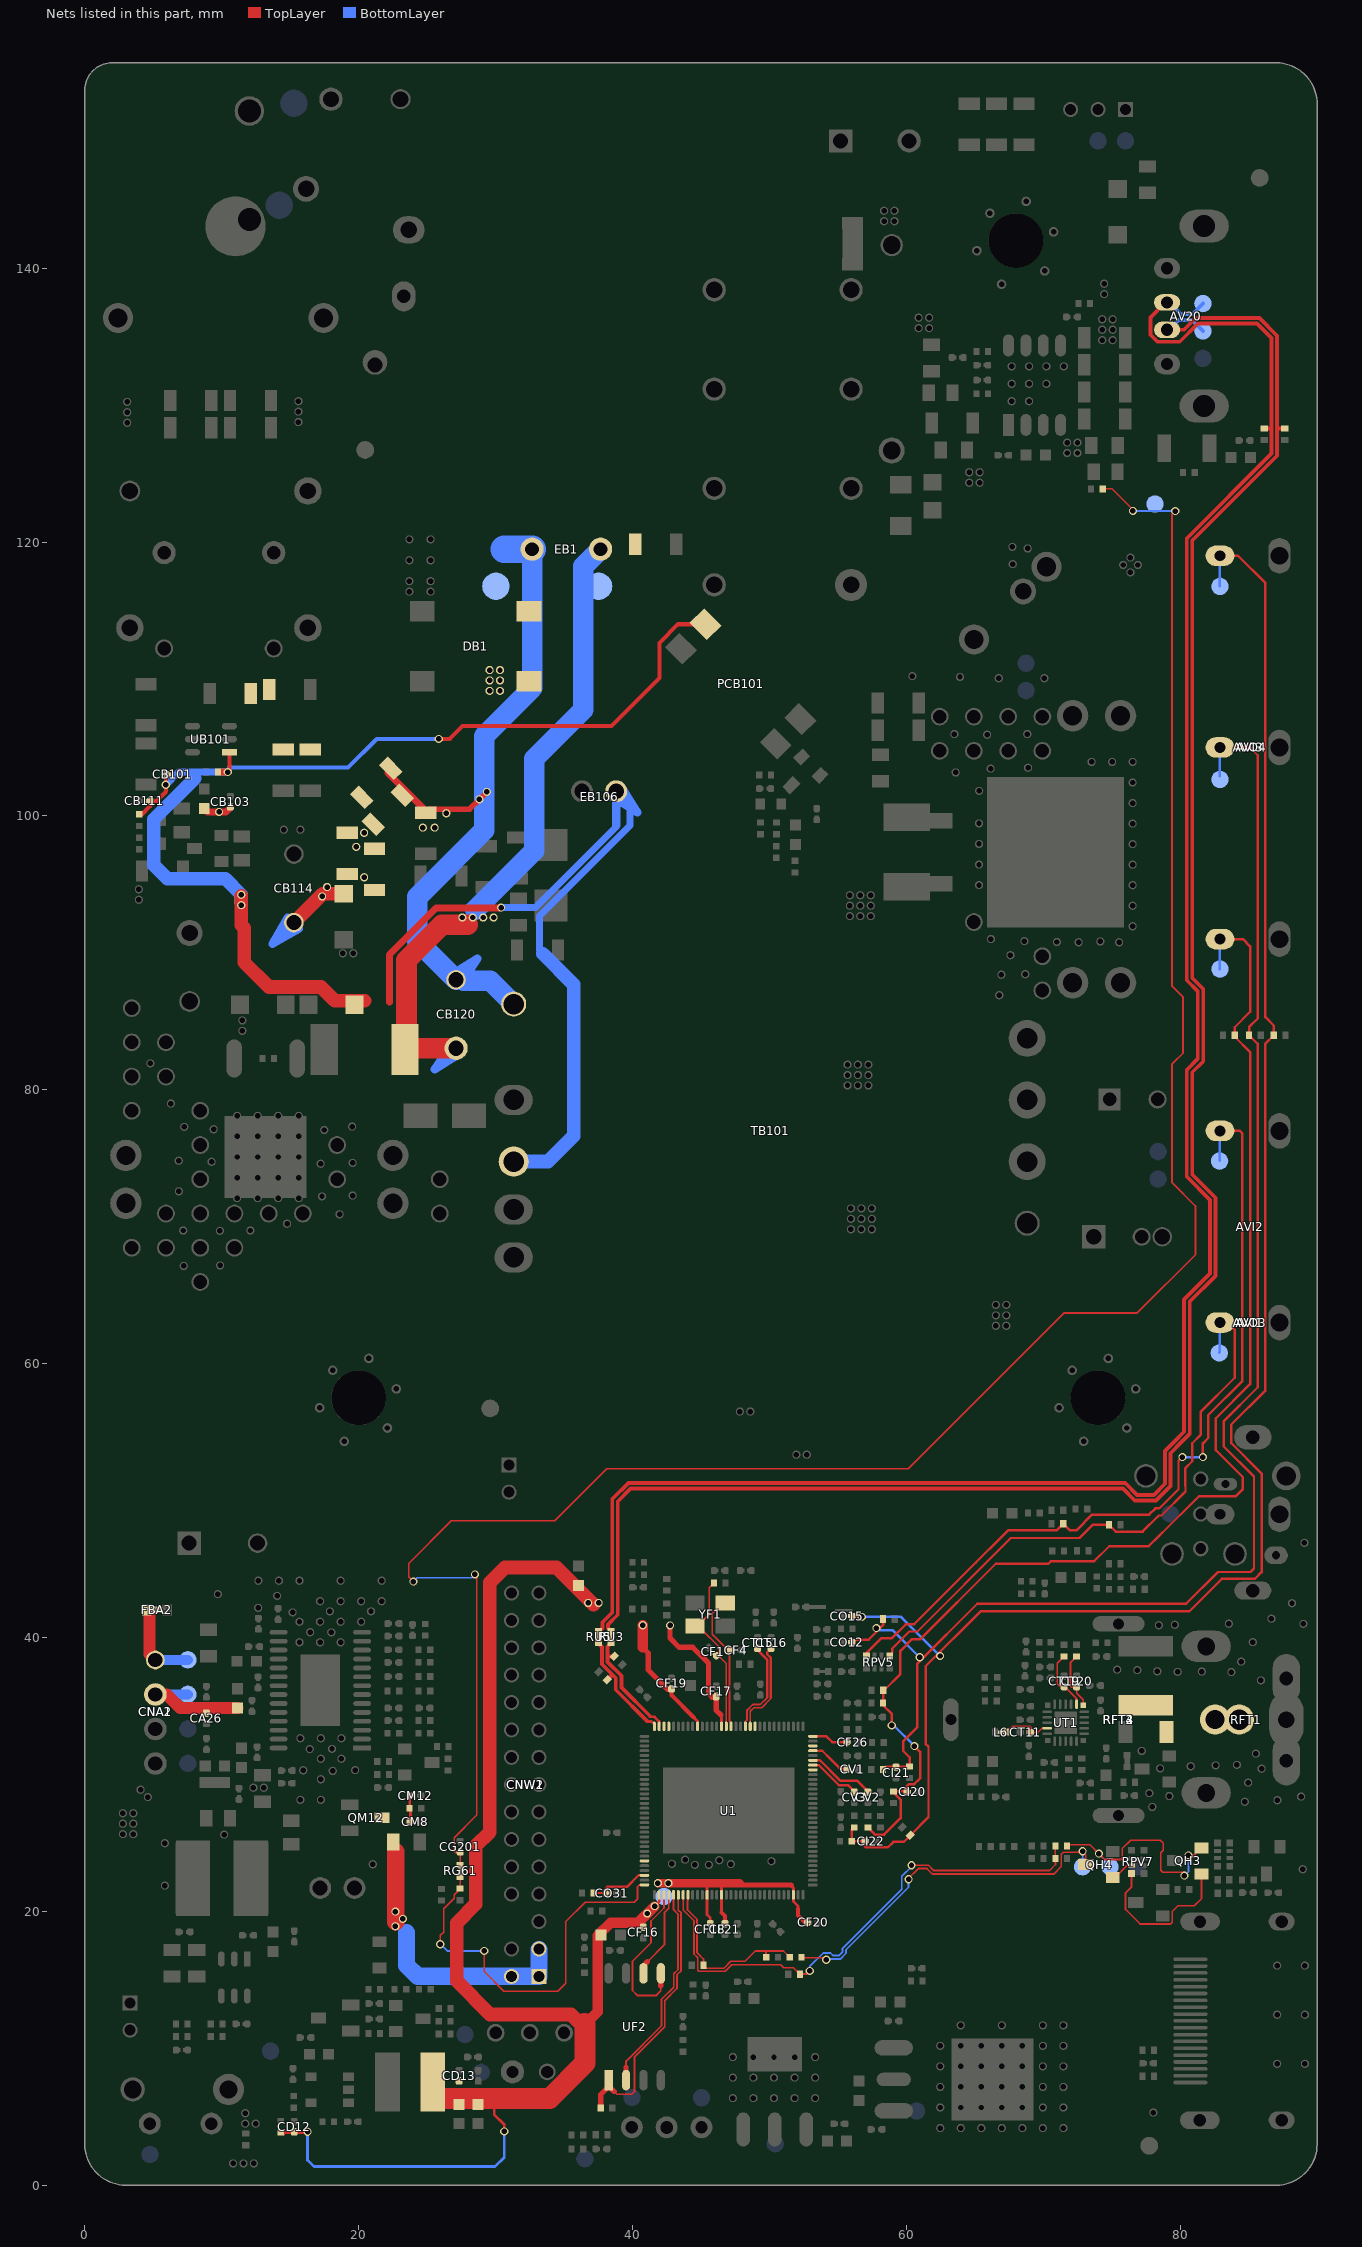
[diagram p0: the nets of this part, all layers, seen from the top]
# Altium PCB MISC116569.PcbDoc (part 12 of 15)
Units mm, origin at the board's own origin, x right, y up, seen from the top; angles counter-clockwise.
Board outline 90 x 155 mm, 2 copper layers (TopLayer, BottomLayer), stack 1.571 mm thick; 527 components, 277 nets, 2450 pads, 649 vias.

## Via types
v1: diameter 0.6, hole 0.4, TopLayer to BottomLayer, tented both sides, 649 vias

## Nets (pads, with @x,y where several pads share a name; then routed paths per layer and width w, separated by ;. In a path a pad name is that pad's centre, name@x,y a point inside that pad or via, vN(x,y) a via of type N, cw(c..) or ccw(c..) an arc to the next point about the centre after c; other vN are vias at no path point) (continued)
PWM1: RF13.1 RG61.1 U1.96 | length 29.4
  TopLayer w0.127: v1(25.967,17.605) 25.967,18.241 26.213,18.487 26.213,19.256 ; 26.213,19.531 26.213,19.256 ; RG61.1@27.414,22.526 RF13.1@27.414,21.662 26.974,21.221 26.974,20.961 26.213,20.2 26.213,19.256 ; v1(29.167,17.109) 29.167,15.605 30.609,14.163 34.533,14.163 35.127,14.757 35.127,19.255 36.546,20.674 40.14,20.674 40.36,20.894 40.36,21.774 40.518,21.932 U1.96@40.873,21.932
  BottomLayer w0.127: v1@25.971,17.605 v1(25.967,17.605) 26.462,17.109 v1(29.167,17.109)
PWM_REF: CG201.1 PWM_REF.1 RB801.1 RG61.2 RG61.3 | length 157.1
  TopLayer w0.127: v1(24.003,44.088) 23.652,44.439 23.652,45.406 26.775,48.529 34.327,48.529 38.122,52.324 60.147,52.324 71.526,63.703 76.867,63.703 81.115,67.951 81.115,71.508 79.408,73.214 79.408,81.888 80.208,82.688 80.208,86.763 79.408,87.563 79.408,122.026 v1(79.645,122.263) ; RG61.2@27.414,23.376 CG201.1@27.414,24.294 ; CG201.1@27.414,24.294 27.075,24.294 26.974,24.395 26.974,25.382 28.624,27.033 v1@28.624,44.608 ; RB801.1@74.34,123.888 75.014,123.888 76.551,122.352 v1(76.551,122.276)
  BottomLayer w0.127: v1(24.003,44.088) 24.287,44.371 28.252,44.371 v1(28.489,44.608) ; v1(76.551,122.276) 79.632,122.276 v1(79.645,122.263)
RF_INPUT: CT3.2 GDT1.1 RFT1.1 RFT2.1@84.3,34 RFT3.1@84.3,34 RFT4.1
ROUT+: CNA1.1 CNA2.1 FBA2.2 FBA2.3 ROUT+.1 | length 6.1
  TopLayer w0.889: FBA2.2@4.609,41.872 4.734,41.747 4.734,38.777 CNA1.1@5.156,38.355
  BottomLayer w0.762: CNA1.1@5.156,38.355 ROUT+.1@7.51,38.355
ROUT-: BA3.2 CA26.2@8.877,34.52 CA26.2@8.877,34.345 CNA1.2 CNA2.2 ROUT-.1 | length 9
  TopLayer w0.762: CNA1.2@5.156,35.835 CNA1.2@5.426,35.835
  TopLayer w0.889: CNA1.2@5.156,35.835 5.982,35.835 6.974,34.842 11.149,34.842 BA3.2@11.151,34.841
  BottomLayer w0.762: CNA1.2@5.156,35.835 ROUT-.1@7.51,35.835
SCL_EN: QH4.B RPV7.5 | length 1.9
  TopLayer w0.127: QH4.B@75.082,22.466 75.235,22.466 76.126,23.358 RPV7.5@76.451,23.358 RPV7.5@76.281,23.358
SDA_EN: QH3.B RPV7.7 | length 11.8
  TopLayer w0.127: RPV7.7@76.451,22.758 76.451,21.787 76.013,21.349 76.013,20.139 77.067,19.084 79.314,19.084 79.426,19.196 79.426,19.993 79.836,20.403 81.026,20.403 81.554,20.932 QH3.B@81.554,22.735
SGND: CB101.2@5.957,103.035 CB101.2@6.132,103.035 CB102.2 CB103.1 CB111.2@4.61,101.098 CB111.2@4.785,101.098 CB120.1 DB1.4 DB110.K EB1.2 EB106.2 pad.VIA5@11.43,93.485 pad.VIA5@11.43,94.247 pad.VIA5@27.572,92.581 pad.VIA5@28.334,92.581 pad.VIA5@29.096,92.581 pad.VIA5@29.858,92.581 PCB101.3 RB103.1 RB104.2 RB130.1 RB148.1 TB101.4 TP-TDT.2 UB101.1 | length 189.8
  TopLayer w0.3: RB103.1@3.975,100.12 4.159,100.12 4.785,100.746 CB111.2@4.785,101.098 ; CB111.2@4.861,101.098 5.252,101.098 5.918,101.764 v1(5.918,102.273) CB101.2@5.918,102.996 ; v1(25.844,105.626) 26.649,105.626 27.599,106.575 38.452,106.575 41.961,110.084 41.961,112.628 43.334,114.002 PCB101.3@45.333,114.002
  TopLayer w0.305: v1(10.444,103.2) 10.558,103.314 UB101.1@10.558,104.65 10.558,103.781
  TopLayer w0.5: CB102.2@8.725,100.538 8.971,100.292 v1(9.804,100.292) 10.306,100.292 CB103.1@10.63,100.616 ; RB104.2@9.881,103.2 v1(10.444,103.2) ; 22.263,86.398 22.263,89.865 25.667,93.269 30.34,93.269 30.353,93.256 v1(30.404,93.307)
  TopLayer w1: pad.VIA5@11.432,94.17 11.432,92.037 11.648,91.821 11.648,89.304 13.452,87.5 17.256,87.5 18.244,86.512 20.434,86.512
  TopLayer w1.5: RB148.1@23.384,82.944 RB148.1@23.475,83.034 ; CB120.1@27.115,83.034 RB148.1@23.475,83.034 ; 27.959,92.062 26.086,92.062 23.495,89.471 23.495,83.054 RB148.1@23.475,83.034
  BottomLayer w0.3: 10.528,103.531 19.229,103.531 21.323,105.626 24.117,105.626 ; 24.701,105.626 24.117,105.626 ; v1(25.844,105.626) 24.117,105.626
  BottomLayer w0.5: v1(5.918,102.273) 6.853,103.208 v1@10.205,103.208 ; v1(30.404,93.307) 32.918,93.307 38.811,99.2 38.811,99.314 ; 33.21,90.183 33.21,92.697 39.807,99.293 39.807,100.49
  BottomLayer w0.6: 38.811,99.314 EB106.2@38.811,101.486
  BottomLayer w1: 8.026,102.743 5.042,99.758 5.042,96.407 6.037,95.412 10.265,95.412 pad.VIA5@11.43,94.247 11.432,94.244 pad.VIA5@11.432,93.65 ; TB101.4@31.323,74.756 33.837,74.756 35.7,76.619 35.7,87.694 33.455,89.938
  BottomLayer w1.5: 28.511,93.154 32.817,97.46 32.817,104.178 36.398,107.759 36.398,118.216 EB1.2@37.666,119.484
SNB-D-: CB114.2 DB106.K pad.VIA5@17.332,94.12 pad.VIA5@17.691,94.805 pad.VIA5@20.396,95.517 RB125.1 RB127.1 | length 4.5
  TopLayer w1: CB114.2@15.269,92.209 17.37,94.31 DB106.K@18.898,94.31
SNB-RM: pad.VIA5@19.825,97.739 pad.VIA5@20.396,98.768 RB125.2 RB126.1 RB127.2 RB128.1
SPDIF_OUT_IC: CO31.2@38.057,21.338 CO31.2@38.232,21.338 RO21.2 U1.94 | length 4.5
  TopLayer w0.178: RO21.2@37.123,21.338 CO31.2@38.057,21.338 38.057,21.669 38.171,21.783 39.602,21.783 40.451,22.632 U1.94@40.873,22.632
  TopLayer w0.203: U1.94@40.873,22.632 U1.94@40.925,22.632
SPI_CLK: U1.100 UF2.6 | length 6.5
  TopLayer w0.127: 41.098,16.329 42.332,17.564 42.332,19.911 42.649,20.228 U1.100@42.649,21.207
  TopLayer w0.381: UF2.6@40.8,15.471 40.8,16.032 41.098,16.329
SPI_CSN: RF3.1 U1.102 UF2.1 | length 20.9
  TopLayer w0.127: UF2.1@38.387,7.318 38.387,7.127 38.87,6.645 39.962,6.645 40.14,6.822 40.14,9.352 42.35,11.561 42.35,13.473 43.243,14.366 43.243,15.353 43.548,15.658 43.548,19.895 43.349,20.094 U1.102@43.349,21.207
  TopLayer w0.381: RF3.1@37.676,5.641 37.676,6.632 38.26,7.216 UF2.1@38.26,7.671 ; UF2.1@38.26,7.241 38.66,6.841
SPI_DI: U1.99 UF2.5 | length 11.6
  TopLayer w0.127: 42.07,14.544 42.07,14.188 41.745,13.863 40.351,13.863 39.995,14.219 39.995,16.362 41.351,17.718 41.351,19.299 42.299,20.246 U1.99@42.299,21.207 ; U1.99@42.3,21.207 U1.99@42.3,21.257
  TopLayer w0.381: 42.07,14.544 UF2.5@42.07,15.471
SPI_DO: U1.101 UF2.2 | length 15.2
  TopLayer w0.127: 39.53,8.638 39.53,9.065 42.121,11.656 42.121,13.567 43.014,14.46 43.014,15.447 43.32,15.753 43.32,19.8 43,20.12 U1.101@42.999,21.207
  TopLayer w0.381: UF2.2@39.53,7.671 39.53,8.638
TUNER_AGC_OUT_IC: U1.43
TUNER_IF_N_IN_IC: CT15.2@49.136,39.18 CT15.2@49.136,39.355 U1.45 | length 6.9
  TopLayer w0.127: U1.45@48.249,33.508 48.249,33.88 48.37,34.001 48.37,34.698 48.777,35.104 49.338,35.104 49.8,35.566 49.8,35.602
  TopLayer w0.178: CT15.2@49.136,39.18 49.136,39.081 49.825,38.392 49.825,35.628
TUNER_IF_P_IN_IC: CT16.1 U1.44 | length 7.1
  TopLayer w0.127: U1.44@48.599,33.508 48.599,34.603 48.871,34.876 49.433,34.876 50.104,35.548 50.104,35.584
  TopLayer w0.178: 50.104,35.584 50.104,38.508 49.843,38.77 49.843,38.918 CT16.1@50.104,39.18 ; CT16.1@50.104,39.292 CT16.1@50.104,39.18 ; CT16.1@50.127,39.087 50.104,39.065 CT16.1@50.104,39.18
TUNER_SCL: CT20.2@72.436,36.369 CT20.2@72.436,36.544 RT15.1 UT1.7 | length 4.3
  TopLayer w0.127: RT15.1@72.436,38.623 71.995,38.183 71.995,36.46 72.086,36.369 CT20.2@72.436,36.369 72.436,36.337 72.436,35.933 72.927,35.443 UT1.7@72.927,35.068
TUNER_SDA: CT19.2@71.521,36.369 CT19.2@71.521,36.544 RT14.1 UT1.8 | length 4.8
  TopLayer w0.127: CT19.2@71.366,36.404 CT19.2@71.556,36.404 ; CT19.2@71.521,36.544 CT19.2@71.521,36.439 ; RT14.1@71.521,38.623 71.014,38.116 71.014,36.617 71.192,36.439 CT19.2@71.521,36.439 ; UT1.8@72.432,35.122 72.432,35.529 CT19.2@71.556,36.404 ; CT19.2@71.521,36.439 CT19.2@71.556,36.404
UART_RX: QH4.C RH89.1 UART_RX.1 | length 27.1
  TopLayer w0.127: RH89.1@52.351,16.632 RH89.1@52.331,16.652 52.379,16.604 v1@54.107,16.604 ; v1@60.16,22.412 60.87,23.122 61.507,23.122 61.907,22.723 70.754,22.723 71.31,23.279 71.31,24.158 ; 71.327,24.192 71.455,24.32 72.873,24.32 73.1,24.093 QH4.C@73.1,23.431
  BottomLayer w0.127: v1@54.209,16.515 55.16,16.515 55.596,16.951 55.596,17.193 60.16,21.757 v1(60.16,22.352) ; UART_RX.1@72.873,23.254 v1(72.873,24.397)
  other v1: 54.153,16.459
UART_RX_IC: D102.K RF9.1 RH89.2 U1.104 | length 13.2
  TopLayer w0.127: U1.104@44.05,21.207 44.05,20.829 44.023,20.802 44.023,20.1 44.717,19.406 44.717,16.98 45.18,16.517 D102.K@45.18,16.081 45.413,15.847 46.682,15.847 47.187,16.352 48.22,16.352 48.973,17.105 49.741,17.105 ; RF9.1@49.773,16.652 49.741,16.684 49.741,17.105 ; RH89.2@51.481,16.652 51.028,17.105 49.741,17.105
UART_TX: QH3.E RH88.2 UART_TX.1 | length 16.2
  TopLayer w0.127: RH88.2@71.73,24.778 71.818,24.867 73.412,24.867 v1(74.063,24.216) 74.498,23.781 75.661,23.781 75.773,23.892 75.773,24.592 76.38,25.199 78.554,25.199 78.764,24.989 78.764,24.471 78.578,24.285 78.578,23.007 78.729,22.856 v1@80.31,22.856 ; v1@80.856,23.942 QH3.E@81.554,24.64
  BottomLayer w0.127: v1(74.063,24.216) UART_TX.1@74.873,23.406 ; v1(80.31,22.608) 80.602,22.901 v1(80.602,24.082)
UART_TX_IC: D101.K RF8.1 RH88.1 U1.103 | length 38.4
  TopLayer w0.127: U1.103@43.699,21.207 43.7,20.1 44.488,19.312 44.488,16.885 44.763,16.611 44.763,15.707 44.851,15.618 46.777,15.618 47.256,16.098 50.824,16.098 51.04,15.881 51.762,15.881 D101.K@52.223,15.42 52.726,15.42 ; v1@60.384,23.376 61.613,23.376 62.012,22.977 70.449,22.977 70.892,23.42 RF8.1@70.892,23.863 ; RF8.1@70.88,23.863 RH88.1@70.88,24.778
  BottomLayer w0.127: v1(52.951,15.645) 52.951,15.981 53.928,16.959 54.459,16.959 54.648,16.769 55.054,16.769 55.342,17.057 55.342,17.298 59.665,21.621 59.665,22.55 60.376,23.262 v1(60.376,23.368)
USB0_DM_IO: AV20.2@79.04,135.5 DM0.1 DU1.K RU3.2 RU3.3 | length 153.4
  TopLayer w0.279: RU3.2@38.431,40.471 38.209,40.693 38.209,40.947 38.925,41.663 38.925,49.938 39.864,50.876 75.816,50.876 76.683,50.009 78.242,50.009 79.291,51.058 79.291,53.454 80.107,54.27 80.691,54.854 80.691,64.515 82.588,66.413 82.588,72.118 80.881,73.825 80.881,81.242 80.881,81.278 81.682,82.078 81.682,87.373 80.881,88.173 80.881,120.105 87.079,126.303 87.079,135.071 85.788,136.362 81.122,136.362 80.26,135.5 AV20.2@79.04,135.5 ; 87.086,128.301 DU1.K@87.625,128.301
  BottomLayer w0.279: AV20.2@79.04,135.5 79.161,135.5 79.891,136.23 80.844,136.23 DM0.1@81.656,135.417
USB0_DM_IO_IC: DU3.K RU3.1 U1.63 | length 8.3
  TopLayer w0.203: 41.274,34.217 41.285,34.206 41.62,34.206 41.949,33.877 U1.63@41.949,33.508
  TopLayer w0.279: 38.246,38.619 DU3.K@38.658,38.619 ; RU3.1@38.431,39.57 38.184,39.323 38.184,38.211 39.187,37.208 39.187,36.357 41.301,34.244
USB0_DP_IO: AV20.3 DP0.1 DU2.K RU5.2 RU5.3 | length 157.4
  TopLayer w0.279: RU5.2@37.518,40.471 37.581,40.471 37.803,40.693 37.803,41.116 38.519,41.832 38.519,50.106 39.696,51.283 75.985,51.283 76.851,50.416 78.073,50.416 78.884,51.227 78.884,53.622 79.578,54.316 80.284,55.022 80.284,64.684 82.182,66.581 82.182,71.95 80.475,73.656 80.475,81.446 81.275,82.246 81.275,87.205 80.475,88.005 80.475,120.274 86.673,126.471 86.673,134.903 85.62,135.956 81.29,135.956 79.968,134.633 78.331,134.633 77.823,135.141 77.823,136.413 78.91,137.5 AV20.3@79.04,137.5 ; DU2.K@86.126,128.301 86.629,128.301
  BottomLayer w0.279: AV20.3@79.04,137.5 79.193,137.5 80.056,136.637 80.876,136.637 DP0.1@81.656,137.417
USB0_DP_IO_IC: DU4.K RU5.1 U1.64 | length 8.5
  TopLayer w0.203: 41.056,33.914 41.094,33.875 41.382,33.875 41.599,33.659 U1.64@41.599,33.508
  TopLayer w0.279: RU5.1@37.518,39.57 37.778,39.31 37.778,38.043 38.501,37.319 ; DU4.K@38.142,36.913 38.501,37.273 38.501,37.319 ; 41.056,33.914 38.781,36.189 38.781,37.04 38.501,37.319
USB1_DM_IO_IC: U1.61
USB1_DP_IO_IC: U1.62
VBL_CTRL: U1.91
VBRIDGE: CB120.2 DB1.1 EB1.1 pad.VIA5@24.689,99.149 pad.VIA5@25.546,99.149 pad.VIA5@26.403,100.19 pad.VIA5@28.824,101.214 pad.VIA5@29.362,101.752 pad.VIA5@29.561,109.131 pad.VIA5@29.561,109.893 pad.VIA5@29.561,110.655 pad.VIA5@30.323,109.131 pad.VIA5@30.323,109.893 pad.VIA5@30.323,110.655 RB117.2 RB118.2 RB126.2 RB128.2 RB161.1 TB101.1 TP-TDT.1 | length 51.2
  TopLayer w0.4: RB161.1@25.119,100.495 28.105,100.495 pad.VIA5@28.824,101.214 pad.VIA5@29.362,101.752
  TopLayer w0.5: RB126.2@22.146,103.152 RB161.1@24.854,100.444
  BottomLayer w1.5: CB120.2@27.114,88.035 24.295,90.854 24.295,94.082 29.159,98.946 29.159,105.816 32.69,109.347 32.69,119.215 EB1.1@32.421,119.484 ; CB120.2@27.66,87.973 29.606,87.973 TB101.1@31.323,86.256
  BottomLayer w2: 30.648,119.484 32.421,119.484 EB1.1@32.666,119.484
VCC_PANEL: CM7.1 CM8.2@23.9,26.53 CM8.2@23.725,26.53 CM12.1 CNW1.1 CNW1.2 CNW1.3 CNW2.1 CNW2.2 CNW2.3 pad.VIA5@22.69,18.91 pad.VIA5@22.69,19.988 pad.VIA5@23.229,19.449 QM12.D RM15.1 VCC_PANEL.1 | length 22.9
  TopLayer w0.203: CM8.2@23.725,26.53 23.794,26.599 RM15.1@23.794,27.533 ; RM15.1@23.726,27.533 CM12.1@23.726,28.448
  TopLayer w1.27: 22.715,19.22 22.715,21.361 ; pad.VIA5@22.715,19.871 22.715,21.361 ; 22.715,24.361 22.715,21.361
  BottomLayer w1.27: 23.496,18.439 23.496,16.072 24.317,15.251 CNW2.2@31.164,15.251 CNW2.1@33.164,15.251 ; CNW2.1@33.167,15.251 CNW2.3@33.167,17.186
VCOM0: CF26.1 U1.32 | length 2.6
  TopLayer w0.178: U1.32@53.175,32.782 54.162,32.782 54.585,32.36 CF26.1@55.646,32.36
VDDC_CORE: CD10.2 CD12.2@15.299,3.845 CD12.2@15.299,4.02 CD13.2@27.338,7.566 CD13.2@27.338,7.741 CD14.2 CD15.2 CF15.2 CF16.2@40.787,18.706 CF16.2@40.787,18.881 CF17.2@46.114,35.641 CF17.2@46.114,35.816 CF18.1 CF19.1 CF20.2@52.762,19.192 CF20.2@52.937,19.192 CF21.1 LD2.1 pad.VIA5@36.762,42.522 pad.VIA5@37.524,42.522 pad.VIA5@41.07,19.843 pad.VIA5@41.613,20.386 pad.VIA5@41.859,22.06 pad.VIA5@42.626,22.06 RD9.1 U1.50 U1.55 U1.98 U1.108 U1.111 U1.126 VDDC_CORE.1 | length 140.4
  TopLayer w0.203: RD9.1@14.308,3.845 RD9.1@14.397,3.845 ; RD9.1@14.308,3.934 RD9.1@14.397,3.845 ; RD9.1@14.52,3.721 RD9.1@14.397,3.845 ; v1(16.269,3.899) 16.215,3.845 RD9.1@14.397,3.845 ; 29.306,6.163 29.789,5.679 ; 29.896,5.69 29.896,6.34 29.896,5.169 30.632,4.432 v1(30.632,3.924) v1@30.578,3.979 ; pad.VIA5@41.593,20.349 41.949,20.705 U1.98@41.949,21.207 ; 44.474,34.162 44.75,33.886 U1.55@44.75,33.507 ; 45.45,21.988 45.45,19.756 45.683,19.523 CF18.1@45.683,19.133 ; 46.5,19.914 46.5,21.887 ; U1.50@46.5,33.507 46.5,34.336 ; 51.515,21.925 51.749,21.691 U1.126@51.749,21.207 51.749,20.727 52.09,20.386 52.09,20.195
  TopLayer w0.305: CF19.1@42.85,36.219 42.85,35.786 44.474,34.162 ; 46.493,19.907 46.746,19.654 CF21.1@46.746,19.133 ; 52.09,20.195 52.09,19.711 52.609,19.192 CF20.2@52.762,19.192
  TopLayer w0.381: 40.741,39.28 41.148,38.873 41.148,37.629 42.558,36.219 CF19.1@42.85,36.219 ; v1(42.743,40.884) 42.743,39.954 43.406,39.291 44.393,39.291 45.544,38.141 45.544,35.924 45.827,35.641 CF17.2@46.114,35.641 46.114,34.678 46.456,34.336 ; 47.843,21.925 51.515,21.925 51.577,21.925 51.605,21.897
  TopLayer w0.508: pad.VIA5@41.854,22.06 pad.VIA5@41.859,22.06
  TopLayer w0.61: pad.VIA5@41.859,22.06 pad.VIA5@42.626,22.06 47.843,22.06
  TopLayer w0.762: LD2.1@25.687,6.352 LD2.1@25.7,6.34 ; 36.565,11.744 37.478,12.656 ; 37.478,12.779 37.478,18.238 38.398,19.158 40.402,19.158 pad.VIA5@41.593,20.349 ; 40.741,39.28 v1(40.741,40.896)
  TopLayer w1.016: 36.338,11.64 35.504,12.474 29.594,12.474 27.165,14.902 27.165,19.137 28.549,20.521 28.549,24.765 29.577,25.792 29.577,44.012 30.678,45.113 34.451,45.113 37.162,42.402
  TopLayer w1.524: LD2.1@25.7,6.34 28.729,6.34 29.896,6.34 33.96,6.34 36.542,8.922 36.542,11.767 36.503,11.806
  BottomLayer w0.203: v1(16.269,3.899) 16.269,1.829 16.739,1.359 29.959,1.359 30.632,2.032 v1(30.632,3.924)
VGA_HS_IN_IC: U1.25
VGA_VS_IN_IC: U1.30
VSTR: RB101.2 RB102.1
XTAL_IN_IC: CF4.2@47.11,39.068 CF4.2@47.285,39.068 U1.48 YF1.3 | length 10.2
  TopLayer w0.127: YF1.3@46.769,42.533 46.59,42.533 45.829,41.773 45.829,40.236 46.998,39.068 CF4.2@47.11,39.068 47.078,39.035 47.078,33.921 47.199,33.799 U1.48@47.199,33.508 U1.48@47.18,33.527
XTAL_OUT: CT11.2@68.933,33.079 CT11.2@69.108,33.079 L6.2 L6.3 UT1.17 | length 3.6
  TopLayer w0.127: L6.2@67.324,33.086 67.757,33.519 69.005,33.519 69.108,33.416 CT11.2@69.108,33.079 69.609,33.079 69.903,33.372 UT1.17@70.282,33.372
XTAL_OUT_IC: CF1.2@46.023,38.788 CF1.2@46.147,38.664 RF25.2 U1.49 YF1.1 | length 12.2
  TopLayer w0.127: YF1.1@44.569,40.833 44.724,40.833 45.601,41.709 45.601,43.62 RF25.2@45.95,43.97 ; YF1.1@44.77,40.642 44.991,40.642 46.355,39.279 46.355,38.873 CF1.2@46.147,38.664 46.284,38.664 46.849,38.099 U1.49@46.849,33.508
Y_PB_LOUT: AVI3.3 AVO4.3 CI21.1 CO12.2@55.896,39.652 CO12.2@56.071,39.652 DV3.K DV8.K RV1.2 RV2.1 Y_Pb_LOUT.1 | length 111.8
  TopLayer w0.178: CO12.2@56.071,39.652 56.27,39.85 57.252,39.85 58.306,40.903 DV8.K@58.306,41.351 ; RV2.1@58.284,30.366 58.498,30.581 RV1.2@60.236,30.581 60.236,31.258 59.767,31.727 59.767,32.143 ; 59.763,32.147 59.763,32.403 60.788,33.427 60.788,38.067 65.181,42.461 80.428,42.461 82.751,44.784 85.123,44.784 85.387,45.048 85.387,51.747 83.167,53.966 83.167,55.778 85.662,58.273 85.662,83.353 DV3.K@85.028,83.988 85.028,84.574 85.662,85.208 85.662,104.429 85.091,105 AVO4.3@82.9,105
  BottomLayer w0.178: v1@57.81,40.541 58.984,40.541 v1(60.974,38.551) ; Y_Pb_LOUT.1@82.9,102.911 AVO4.3@82.9,105
  other v1: 57.81,40.691
Y_PR_ROUT: AVI3.5 AVO4.5 CI22.1 CO15.2@55.897,41.557 CO15.2@56.072,41.557 DV5.K DV9.K RV5.2 RV10.1 Y_Pr_ROUT.1 | length 135.4
  TopLayer w0.178: CO15.2@56.072,41.557 v1@56.699,41.557 ; RV10.1@56.195,26.133 56.007,25.945 RV5.2@56.007,25.121 CI22.1@56.95,25.121 ; CI22.1@56.962,25.121 CI22.1@56.962,25.133 CI22.1@56.95,25.121 ; AVO4.5@82.9,119 84.22,119 86.221,116.999 86.221,85.302 86.832,84.692 DV5.K@86.832,83.988 86.221,83.377 86.221,58.042 83.726,55.546 83.726,54.198 85.946,51.978 85.946,44.78 85.442,44.276 83.033,44.276 80.659,41.902 65.413,41.902 61.409,37.897 61.409,32.234 61.616,32.026 61.616,26.882 DV9.K@60.287,25.552 59.812,25.078 59.054,25.078 58.644,24.667 57.066,24.667 56.95,24.784 CI22.1@56.95,25.121
  BottomLayer w0.178: v1@56.828,41.427 v1(56.749,41.507) ; v1@56.896,41.654 v1(56.749,41.507) ; v1(62.466,38.649) 59.688,41.427 59.608,41.507 v1(56.749,41.507) ; Y_Pr_ROUT.1@82.901,116.766 AVO4.5@82.9,119
Y_Y_AV_OUT: AVI3.1 AVO4.1 CI20.1 DV4.K DV7.K RO17.2 RV3.2 RV4.1 Y_Y_AV_OUT.1 | length 97.3
  TopLayer w0.152: 78.489,47.455 78.507,47.455 81.376,50.324
  TopLayer w0.178: RV4.1@57.188,26.112 57.701,25.599 58.37,25.599 59.584,26.814 59.584,28.16 59.182,28.562 59.182,28.695 RV3.2@59.118,28.759 ; v1(58.941,33.579) 58.941,34.402 58.312,35.031 DV7.K@58.312,36.144 58.389,36.144 59.569,37.324 59.569,39.025 60.423,39.88 61.02,39.88 66.526,45.386 66.764,45.386 ; RV3.2@59.055,28.759 RV3.2@59.118,28.759 ; CI20.1@60.109,28.815 CI20.1@60.021,28.727 ; v1(60.588,32.067) 61.007,31.648 61.007,29.71 ; 60.996,29.71 60.576,29.29 60.203,29.29 60.021,29.108 CI20.1@60.021,28.727 ; 67.448,45.386 66.764,45.386 ; 71.36,45.564 71.45,45.564 ; 73.511,45.564 73.025,45.564 ; 78.679,47.645 78.489,47.455 77.696,46.662 74.813,46.662 73.714,45.564 73.025,45.564 ; 81.394,50.324 84.069,50.324 84.583,50.837 84.583,51.702 82.609,53.676 82.609,56.009 85.104,58.505 85.104,82.748 83.98,83.871 DV4.K@83.98,83.988 83.98,84.572 85.104,85.695 85.104,90.477 84.581,91 AVO4.1@82.9,91 ; RV3.2@59.118,28.759 59.99,28.759 CI20.1@60.021,28.727 ; 66.764,45.386 70.377,45.386 70.554,45.564 71.45,45.564 ; 71.45,45.564 73.025,45.564
  BottomLayer w0.178: v1@59.076,33.579 v1(60.588,32.067) ; Y_Y_AV_OUT.1@82.901,88.814 AVO4.1@82.9,91
YPBPR_L/AV_L: AVI1.3 AVI2.1 AVO3.3 DI3.K RPV5.8 YPBPR_L/AV_L.1 | length 44.1
  TopLayer w0.152: RPV5.8@58.685,38.649 58.972,38.935 58.972,39.201 60.197,40.426 60.794,40.426 67.636,47.268 67.654,47.268 ; 78.357,48.831 78.443,48.917 78.64,48.917 80.383,50.66 80.383,51.095
  TopLayer w0.178: 67.654,47.268 72.65,47.268 73.606,48.224 DI3.K@74.792,48.224 75.287,47.729 77.255,47.729 78.357,48.831 ; 80.383,51.095 80.383,52.376 80.882,52.875 80.882,54.191 81.491,54.799 81.491,56.472 83.986,58.967 83.986,62.461 83.447,63 AVI2.1@82.9,63
  BottomLayer w0.178: YPBPR_L/AV_L.1@82.85,60.785 82.9,60.835 AVI2.1@82.9,63
YPBPR_R/AV_R: AVI1.5 AVI2.3 AVO3.5 DI1.K RPV5.2 YPBPR_R/AV_R.1 | length 61.7
  TopLayer w0.152: 78.448,49.425 78.466,49.425 79.875,50.834 79.875,51.107
  TopLayer w0.178: RPV5.2@57.086,38.649 57.086,38.858 58.181,39.953 58.951,39.953 59.971,40.972 60.568,40.972 65.07,45.474 66.984,47.388 ; 67.066,47.47 66.984,47.388 ; 73.764,48.969 74.066,48.969 ; 78.448,49.425 78.189,49.425 77.733,48.969 74.066,48.969 ; 79.875,51.107 79.875,52.885 v1(80.163,53.173) ; v1@81.504,53.33 v1(81.656,53.177) 81.656,54.174 82.05,54.568 82.05,56.241 84.545,58.736 84.545,76.816 84.361,77 AVI2.3@82.9,77 ; 66.984,47.388 67.422,47.827 70.972,47.827 DI1.K@71.458,48.313 71.945,47.827 72.418,47.827 73.561,48.969 74.066,48.969
  BottomLayer w0.178: v1(80.163,53.173) 81.652,53.173 v1(81.656,53.177) ; YPBPR_R/AV_R.1@82.9,74.818 AVI2.3@82.9,77
YPP_Pb&B_IN_IC: CV3.2@56.197,28.584 CV3.2@56.197,28.759 U1.26 | length 3.8
  TopLayer w0.178: U1.26@53.175,30.682 53.605,30.682 55.066,29.221 55.735,29.221 CV3.2@56.197,28.759
YPP_Pr&R_IN_IC: CV1.2@55.637,30.366 CV1.2@55.812,30.366 U1.29 | length 3
  TopLayer w0.127: U1.29@53.175,31.732 53.64,31.732
  TopLayer w0.178: 53.64,31.732 53.855,31.732 54.465,31.123 55.222,30.366 CV1.2@55.637,30.366
YPP_Y&G_IN_IC: CV2.2@57.188,28.584 CV2.2@57.188,28.759 U1.27 | length 5
  TopLayer w0.183: U1.27@53.175,31.032 53.69,31.032 55.194,29.528 56.419,29.528 CV2.2@57.188,28.759